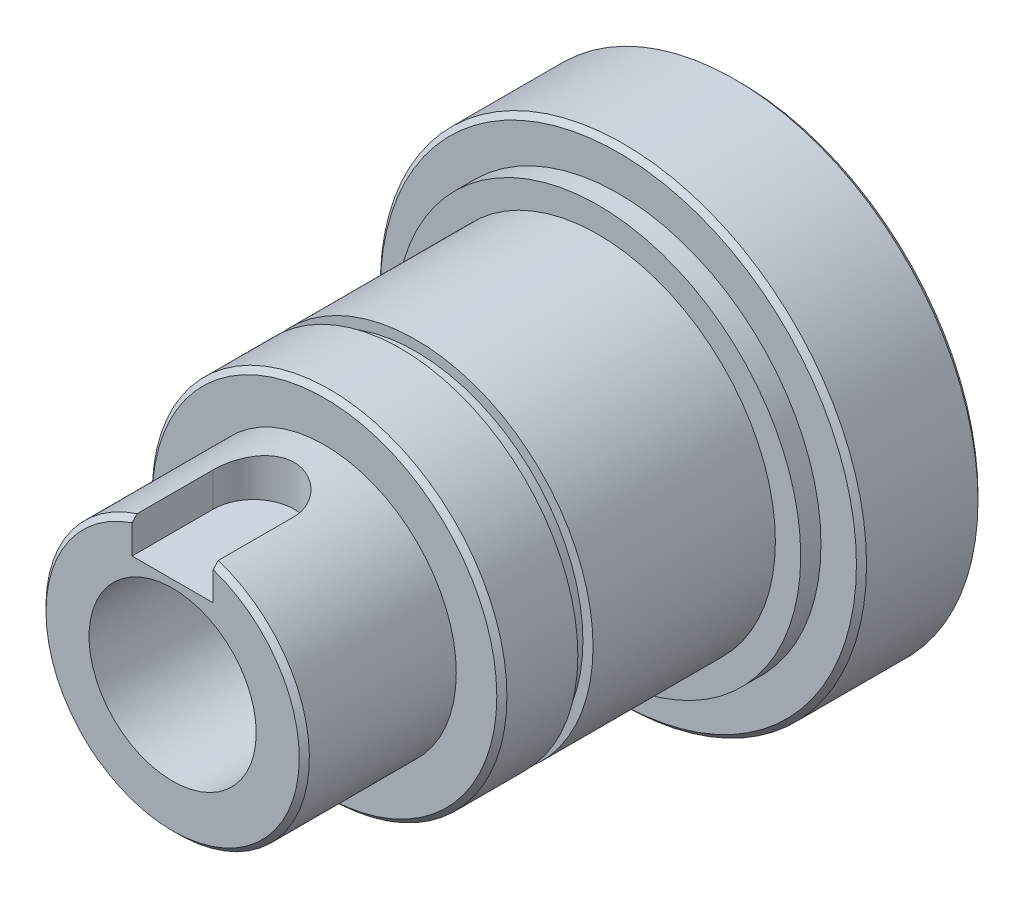
from build123d import *

# Parameters (mm, degrees)
SKETCH1_R             = 24
BOSS_EXTRUDE1_DEPTH   = 12
SKETCH2_R             = 20
BOSS_EXTRUDE2_DEPTH   = 2
SKETCH3_R             = 17.5
BOSS_EXTRUDE3_DEPTH   = 27
SKETCH4_R             = 13
BOSS_EXTRUDE4_DEPTH   = 15
SKETCH5_R             = 14
CUT_EXTRUDE1_DEPTH    = 37.1
SKETCH6_R             = 8.25
CUT_EXTRUDE2_DEPTH    = 66.482822175
CUT_EXTRUDE3_DEPTH    = 4
CUT_EXTRUDE4_START    = -7.5
SKETCH8_R             = 29.21642444
SKETCH8_R_2           = 16.5
CUT_EXTRUDE4_DEPTH    = 1.5
M5_TAPPED_HOLE1_D     = 4.2
M5_TAPPED_HOLE1_DEPTH = 10
M5_TAPPED_HOLE1_TIP   = 1.2618073
CHAMFER1_SIZE         = 0.5


with BuildPart() as part:
    # Sketch1 → Boss-Extrude1 (new body)
    with BuildSketch(Plane.XY):
        Circle(SKETCH1_R)
    extrude(amount=BOSS_EXTRUDE1_DEPTH)

    # Sketch2 → Boss-Extrude2 (add)
    with BuildSketch(Plane.XY.offset(12)):
        Circle(SKETCH2_R)
    extrude(amount=BOSS_EXTRUDE2_DEPTH)

    # Sketch3 → Boss-Extrude3 (add)
    with BuildSketch(Plane.XY.offset(14)):
        Circle(SKETCH3_R)
    extrude(amount=BOSS_EXTRUDE3_DEPTH)

    # Sketch4 → Boss-Extrude4 (add)
    with BuildSketch(Plane.XY.offset(41)):
        Circle(SKETCH4_R)
    extrude(amount=BOSS_EXTRUDE4_DEPTH)

    # Sketch5 → Cut-Extrude1 (cut)
    with BuildSketch(Plane(origin=(0, 0, 0), x_dir=(-1, 0, 0), z_dir=(0, 0, -1))):
        Circle(SKETCH5_R)
    extrude(amount=-CUT_EXTRUDE1_DEPTH, mode=Mode.SUBTRACT)

    # Sketch6 → Cut-Extrude2 (cut, through all)
    with BuildSketch(Plane.XY.offset(56)):
        Circle(SKETCH6_R)
    extrude(amount=-CUT_EXTRUDE2_DEPTH, mode=Mode.SUBTRACT)

    # Sketch7 → Cut-Extrude3 (cut)
    with BuildSketch(Plane(origin=(0, 13, 0), x_dir=(1, 0, 0), z_dir=(0, 1, 0))):
        with BuildLine():
            Line((4, -48), (4, -64))
            ThreePointArc((4, -64), (0, -68), (-4, -64))
            Line((-4, -64), (-4, -48))
            ThreePointArc((-4, -48), (0, -44), (4, -48))
        make_face()
    extrude(amount=-CUT_EXTRUDE3_DEPTH, mode=Mode.SUBTRACT)

    # Sketch8 → Cut-Extrude4 (cut)
    with BuildSketch(Plane.XY.offset(41).offset(CUT_EXTRUDE4_START)):
        Circle(SKETCH8_R)
        Circle(SKETCH8_R_2, mode=Mode.SUBTRACT)
    extrude(amount=-CUT_EXTRUDE4_DEPTH, mode=Mode.SUBTRACT)

    # M5 Tapped Hole1
    with Locations(Plane(origin=(0, 0, 0), x_dir=(-1, 0, 0), z_dir=(0, 0, -1))):
        with Locations((0, 19), (-13.435028843, 13.435028843), (13.435028843, 13.435028843), (-13.435028843, -13.435028843), (0, -19), (13.435028843, -13.435028843)):
            Hole(M5_TAPPED_HOLE1_D / 2, depth=M5_TAPPED_HOLE1_DEPTH)
            with Locations((0, 0, -(M5_TAPPED_HOLE1_DEPTH + M5_TAPPED_HOLE1_TIP / 2))):  # 118° drill point
                Cone(0, M5_TAPPED_HOLE1_D / 2, M5_TAPPED_HOLE1_TIP, mode=Mode.SUBTRACT)

    # Chamfer1
    chamfer1_edges = [part.edges().sort_by_distance(p)[0] for p in [
        (-17.5, 0, 41),
        (-24, 0, 0),
        (-7.64852927, -10.511898021, 56),
        (-24, 0, 12),
    ]]
    chamfer(chamfer1_edges, length=CHAMFER1_SIZE)


solid = part.part
